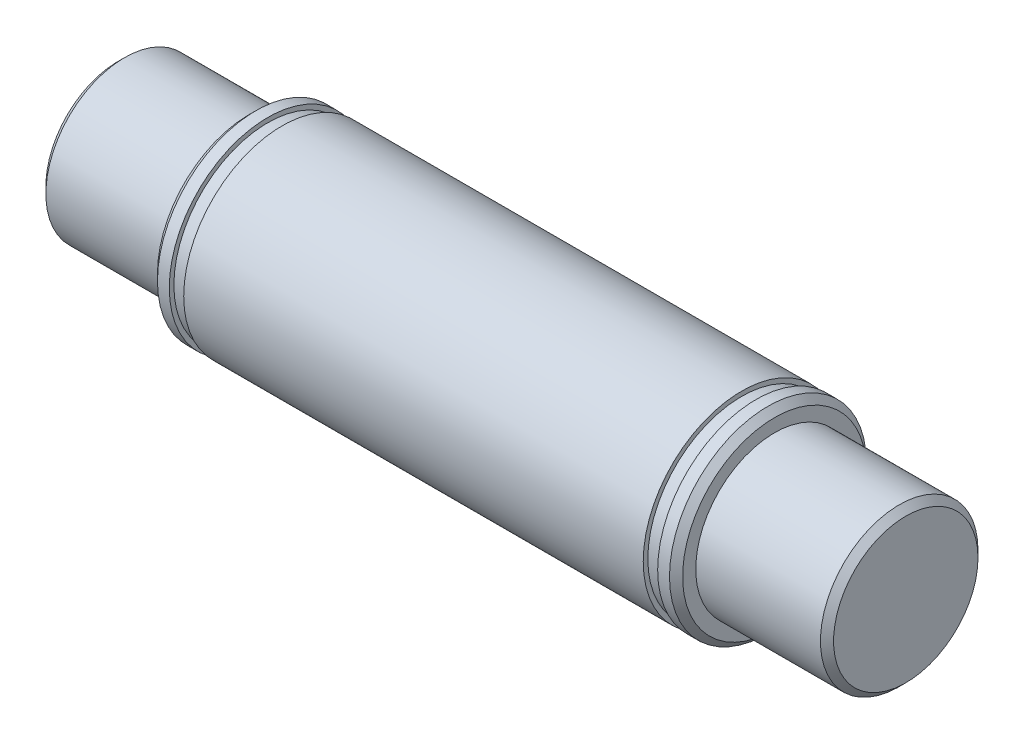
from build123d import *

# Parameters (mm, degrees)
SKETCH_1_R          = 7.5
EXTRUDE_1_DEPTH     = 30
SKETCH_2_OUTSIDE_W  = 29.728
SKETCH_2_OUTSIDE_H  = 29.728
SKETCH_2_OUTSIDE_R  = 6
CUT_EXTRUDE_1_DEPTH = 10
CHAMFER_1_SIZE      = 0.5
SKETCH_3_W          = 1.1
SKETCH_3_H          = 0.35


with BuildPart() as part:
    # 草图1 → 凸台-拉伸1 (new, symmetric)
    with BuildSketch(Plane(origin=(0, 0, 0), x_dir=(0, 0, -1), z_dir=(1, 0, 0))):
        Circle(SKETCH_1_R)
    extrude(amount=EXTRUDE_1_DEPTH, both=True)

    # 草图2 outside → 切除-拉伸1 (cut)
    with BuildSketch(Plane(origin=(30, 0, 0), x_dir=(0, 0, -1), z_dir=(1, 0, 0))):
        Rectangle(SKETCH_2_OUTSIDE_W, SKETCH_2_OUTSIDE_H)
        Circle(SKETCH_2_OUTSIDE_R, mode=Mode.SUBTRACT)
    cut_extrude_1 = extrude(amount=-CUT_EXTRUDE_1_DEPTH, mode=Mode.SUBTRACT)

    # 镜向1: 切除-拉伸1 across plane
    add(cut_extrude_1.mirror(Plane(origin=(0, 0, 0), x_dir=(0, 0, 1), z_dir=(1, 0, 0))), mode=Mode.SUBTRACT)

    # 倒角1
    chamfer_1_edges = [part.edges().sort_by_distance(p)[0] for p in [
        (30, 0, 6),
        (-30, 0, 6),
        (-20, 0, 7.5),
        (20, 0, 7.5),
    ]]
    chamfer(chamfer_1_edges, length=CHAMFER_1_SIZE)

    # 草图3 → 切除-旋转1 (revolve, cut)
    with BuildSketch(Plane.XY, mode=Mode.PRIVATE) as cut_revolve_1_sk:
        with Locations((-18.05, -7.325)):
            Rectangle(SKETCH_3_W, SKETCH_3_H)
    cut_revolve_1 = revolve(cut_revolve_1_sk.sketch.rotate(Axis((-31.365791293, 0, 0), (1, 0, 0)), 270), axis=Axis((-31.365791293, 0, 0), (1, 0, 0)), mode=Mode.SUBTRACT)

    # 镜向2: 切除-旋转1 across plane
    add(cut_revolve_1.mirror(Plane(origin=(0, 0, 0), x_dir=(0, 0, 1), z_dir=(1, 0, 0))), mode=Mode.SUBTRACT)


solid = part.part
